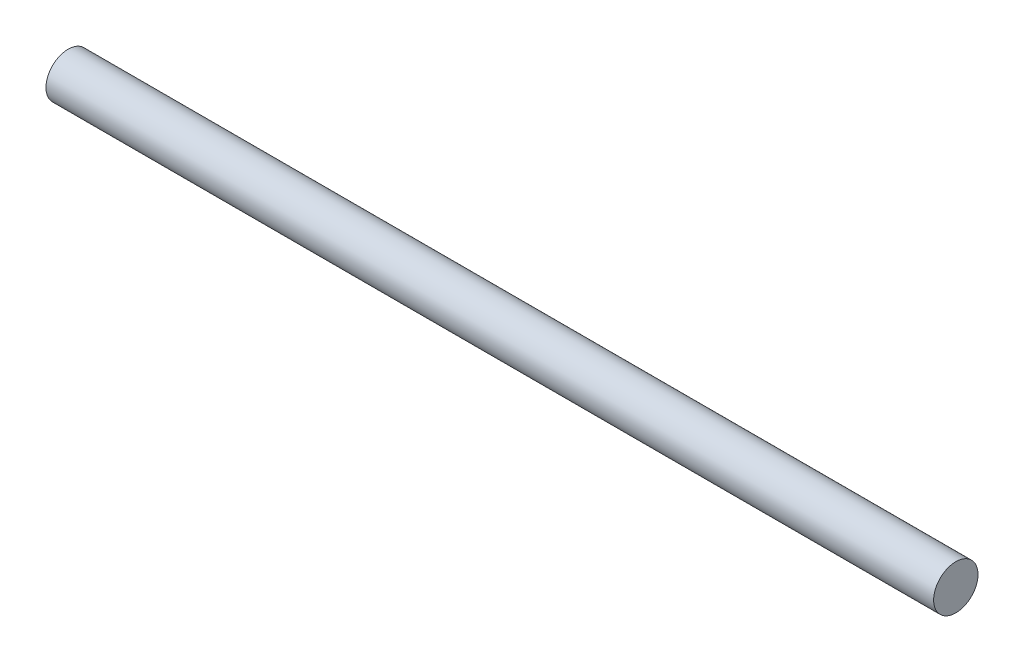
from build123d import *

# Parameters (mm, degrees)
SKETCH1_R    = 20
LENGTH_DEPTH = 800


with BuildPart() as part:
    # Sketch1 → Length (new body)
    with BuildSketch(Plane(origin=(0, 0, 0), x_dir=(0, 0, -1), z_dir=(1, 0, 0))):
        Circle(SKETCH1_R)
    extrude(amount=LENGTH_DEPTH)


solid = part.part
